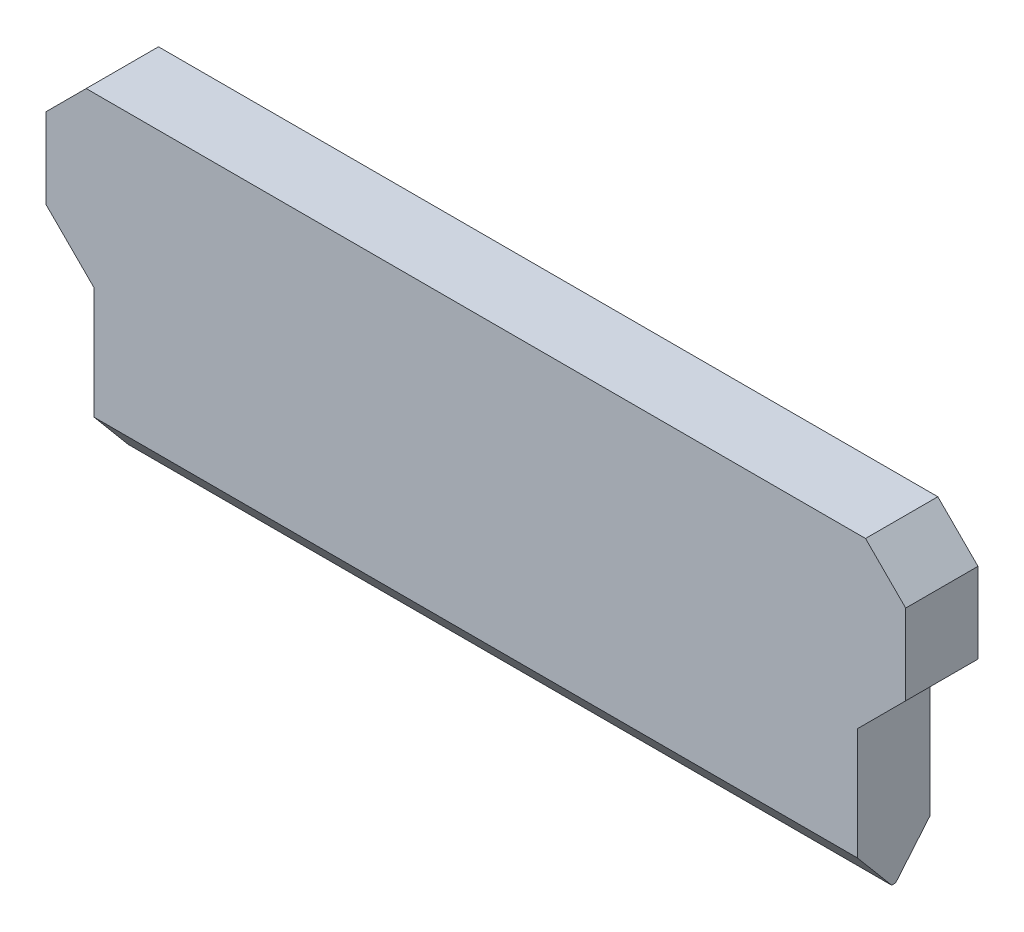
from build123d import *

# Parameters (mm, degrees)
BOSS_EXTRUDE1_DEPTH = 18
CUT_EXTRUDE1_DEPTH  = 214


with BuildPart() as part:
    # Sketch1 → Boss-Extrude1 (new, symmetric)
    with BuildSketch(Plane.XY):
        Polygon((-194, 80), (194, 80), (214, 60), (214, 20), (190, -4), (190, -80), (-190, -80), (-190, -4), (-214, 20), (-214, 60), align=None)
    extrude(amount=BOSS_EXTRUDE1_DEPTH, both=True)

    # Sketch2 → Cut-Extrude1 (cut, symmetric)
    with BuildSketch(Plane(origin=(0, 0, 0), x_dir=(0, 0, -1), z_dir=(1, 0, 0))):
        Polygon((-1, -80), (-18, -59.740188926), (-18, -80), align=None)
        Polygon((1, -80), (18, -59.740188926), (18, -80), align=None)
    extrude(amount=CUT_EXTRUDE1_DEPTH, both=True, mode=Mode.SUBTRACT)


solid = part.part
